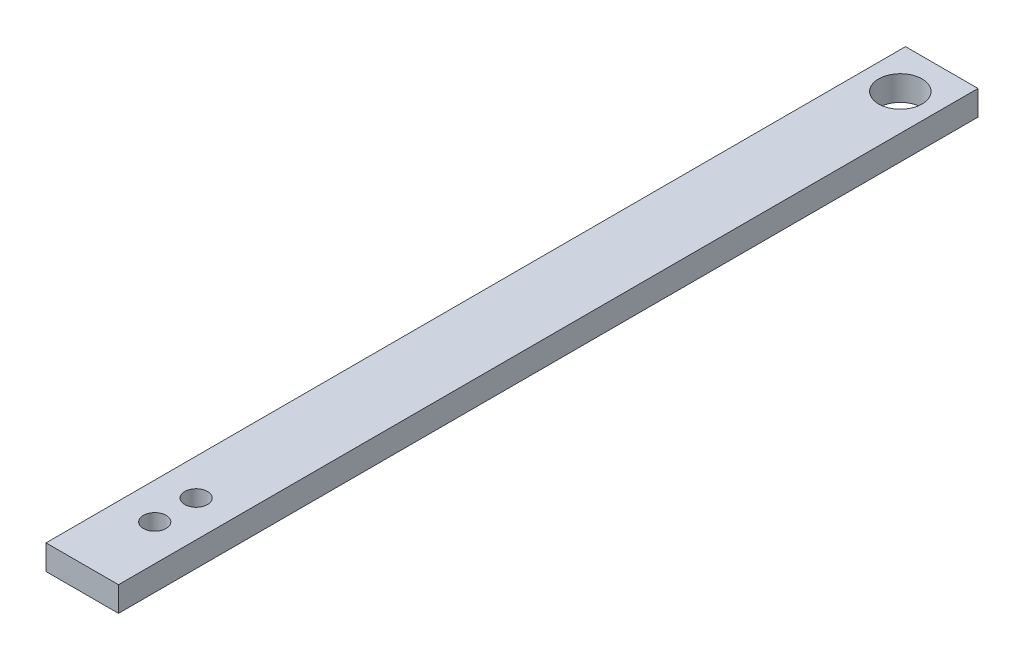
from build123d import *

# Parameters (mm, degrees)
SKETCH_1_W          = 35
SKETCH_1_H          = 12
EXTRUDE_1_DEPTH     = 207.5
SKETCH_2_R          = 10.5
SKETCH_2_R_2        = 5.5
CUT_EXTRUDE_1_DEPTH = 12


with BuildPart() as part:
    # 草图1 → 凸台-拉伸1 (new, symmetric)
    with BuildSketch(Plane.XY):
        Rectangle(SKETCH_1_W, SKETCH_1_H)
    extrude(amount=EXTRUDE_1_DEPTH, both=True)

    # 草图2 → 切除-拉伸1 (cut)
    with BuildSketch(Plane(origin=(0, 6, 0), x_dir=(1, 0, 0), z_dir=(0, 1, 0))):
        with Locations(Location((0, 187.5, 0), (0, 0, 270))):
            Circle(SKETCH_2_R)
        with Locations(Location((0, -152.5, 0), (0, 0, 270))):
            Circle(SKETCH_2_R_2)
        with Locations(Location((0, -172.5, 0), (0, 0, 270))):
            Circle(SKETCH_2_R_2)
    extrude(amount=-CUT_EXTRUDE_1_DEPTH, mode=Mode.SUBTRACT)


solid = part.part
